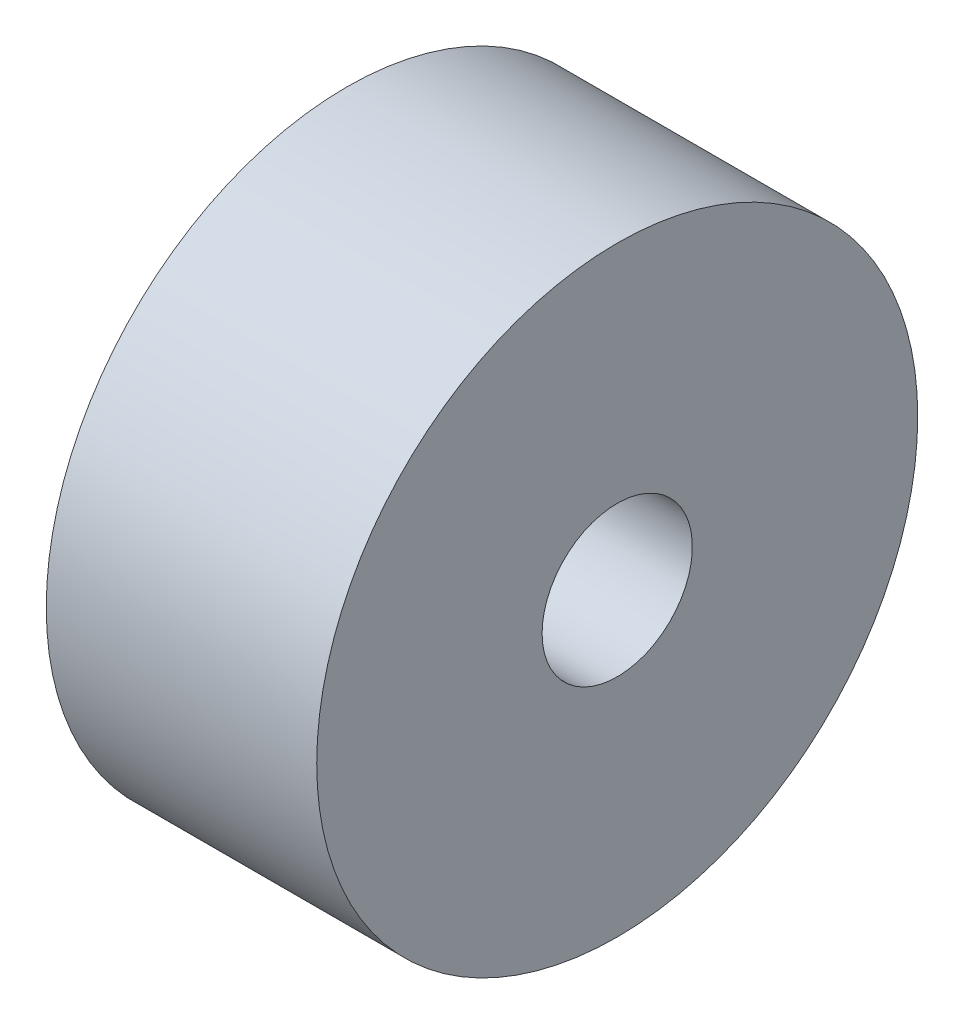
SolidWorks part; units mm, degrees
ref_plane "Front Plane" through (0, 0, 0) normal (0, 0, 1) x (1, 0, 0)
ref_plane "Top Plane" through (0, 0, 0) normal (0, 1, 0) x (1, 0, 0)
ref_plane "Right Plane" through (0, 0, 0) normal (1, 0, 0) x (0, 0, -1)
other "Configuration Table"
sketch "Sketch1" plane through (0, 0, 0) normal (0, 0, 1) x (1, 0, 0)
  line L1 (-109.7137, 0) -> (134.0213, 0) construction
  line L3 (-18, 40) -> (18, 40)
  line L4 (-18, 40) -> (-18, 10)
  line L5 (-18, 10) -> (18, 10)
  line L6 (18, 40) -> (18, 10)
  line L7 (-18, 40) -> (18, 10) construction
  line L8 (-18, 10) -> (18, 40) construction
  dimension "D1" = 30
  dimension "D2" = 36
revolve "Revolve1" add sketch "Sketch1" angle 360 about L1
